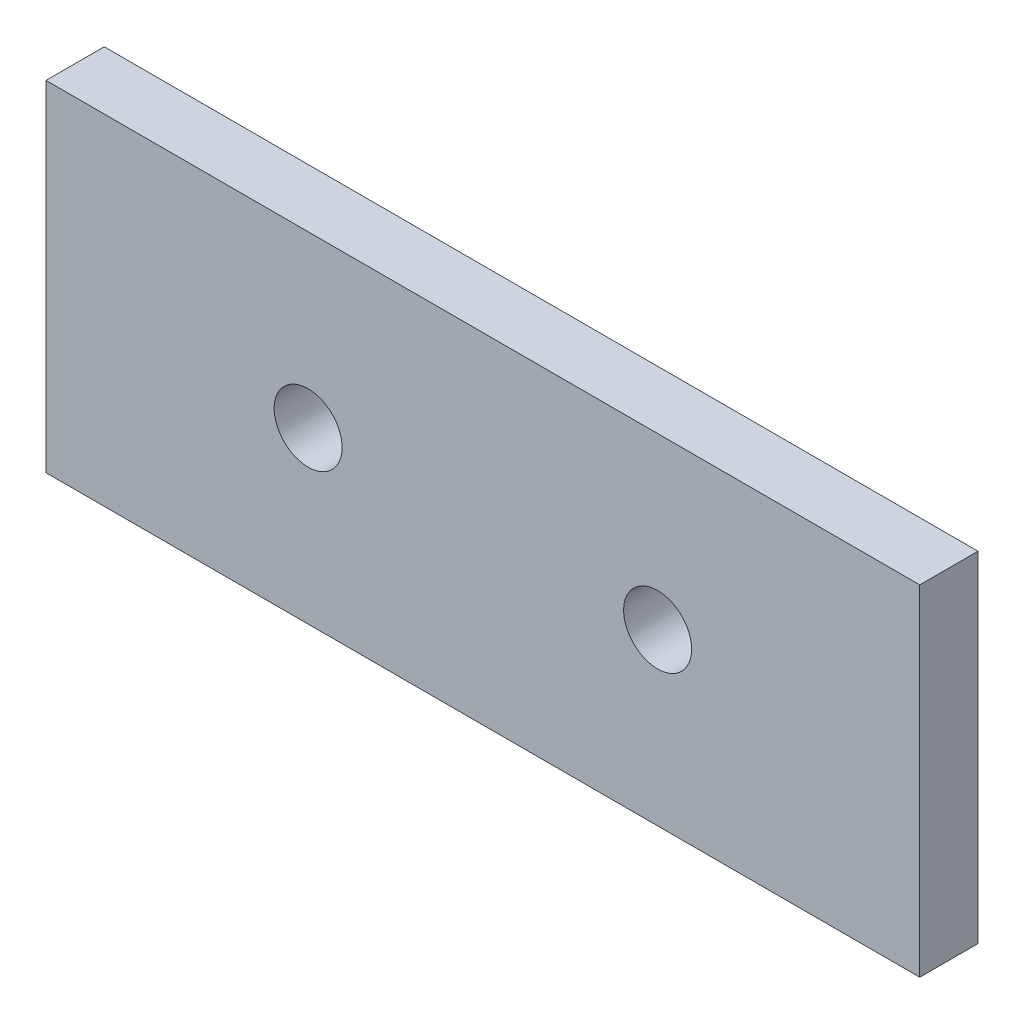
from build123d import *

# Parameters (mm, degrees)
SKETCH1_W            = 90
SKETCH1_H            = 35
BOSS_EXTRUDE1_DEPTH  = 6
M6_CLEARANCE_HOLE1_D = 7


with BuildPart() as part:
    # Sketch1 → Boss-Extrude1 (new body)
    with BuildSketch(Plane.XY):
        with Locations((45, 17.5)):
            Rectangle(SKETCH1_W, SKETCH1_H)
    extrude(amount=BOSS_EXTRUDE1_DEPTH)

    # M6 Clearance Hole1 (through all)
    with Locations(Plane.XY.offset(6)):
        with Locations((27, 17.5), (63, 17.5)):
            Hole(M6_CLEARANCE_HOLE1_D / 2)


solid = part.part
